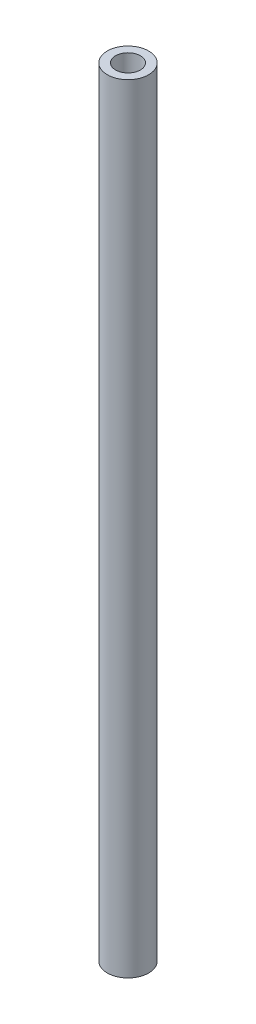
SolidWorks part; units mm, degrees
material "黄铜"
ref_plane "Front Plane" through (0, 0, 0) normal (0, 0, 1) x (1, 0, 0)
ref_plane "Top Plane" through (0, 0, 0) normal (0, 1, 0) x (1, 0, 0)
ref_plane "Right Plane" through (0, 0, 0) normal (1, 0, 0) x (0, 0, -1)
sketch "Sketch1" plane through (0, 0, 0) normal (0, 0, 1) x (1, 0, 0)
  line L0 (0, 23.6464) -> (0, 0) construction
  line L1 (-0.3, 18.84) -> (-0.3, 0)
  line L2 (-0.5, 18.84) -> (-0.3, 18.84)
  line L3 (-0.5, 0) -> (-0.3, 0)
  line L5 (-0.5, 18.84) -> (-0.5, 0)
  dimension "D1" = 0.2
  dimension "D3" = 1
revolve "Revolve2" add sketch "Sketch1" angle 360 about L0
